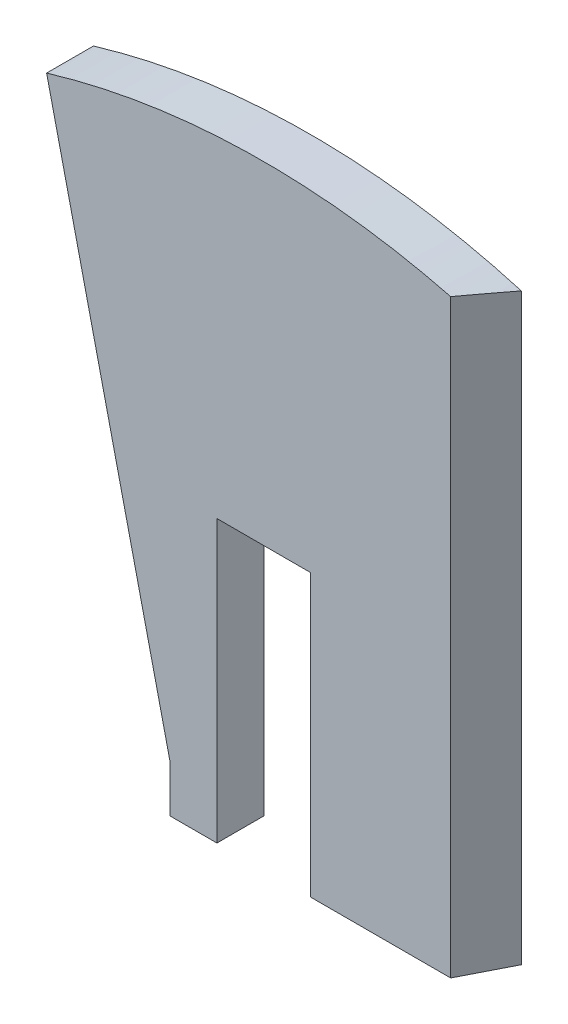
SolidWorks part; units mm, degrees
ref_plane "Front Plane" through (0, 0, 0) normal (0, 0, 1) x (1, 0, 0)
ref_plane "Top Plane" through (0, 0, 0) normal (0, 1, 0) x (1, 0, 0)
ref_plane "Right Plane" through (0, 0, 0) normal (1, 0, 0) x (0, 0, -1)
sketch "Sketch1" plane through (0, 0, 0) normal (0, 0, 1) x (1, 0, 0)
  line L0 (0, 161) -> (0, -161) construction
  line L1 (-46.3607, 154.1807) -> (-20, 40)
  line L2 (-20, 40) -> (-20, 30)
  line L4 (45, 30) -> (45, 40)
  line L5 (45, 40) -> (45, 154.5833)
  line L6 (-20, 30) -> (0, 30)
  line L7 (0, 30) -> (45, 30)
  line L8 (45, 154.5833) -> (0, 30) construction
  arc A0 (45, 154.5833) -> (-46.3607, 154.1807) centre (0, 0) ccw
  dimension "D3" = 322
  dimension "D1" = 30
  dimension "D2" = 20
  dimension "D4" = 10
  dimension "D5" = 45
  dimension "D6" = 13
extrude "Boss-Extrude1" add sketch "Sketch1" along normal mid plane 10
sketch "Sketch2" plane through (0, 0, 5) normal (0, 0, 1) x (1, 0, 0)
  line L0 (-20, 30) -> (45, 30) construction
  line L1 (10, -30) -> (-10, -30)
  line L2 (10, -30) -> (10, 90)
  line L3 (10, 90) -> (-10, 90)
  line L4 (-10, -30) -> (-10, 90)
  line L5 (10, -30) -> (-10, 90) construction
  line L6 (10, 90) -> (-10, -30) construction
  line L7 (-20, 40) -> (-20, 30) construction
  point P0 (0, 30)
  dimension "D1" = 10
  dimension "D2" = 20
  dimension "D3" = 60
extrude "Cut-Extrude1" cut sketch "Sketch2" against normal blind 10
sketch "Sketch3" plane through (0, 30, 0) normal (0, -1, 0) x (1, 0, 0)
  line L4 (45, -5) -> (39.9047, 5)
  line L5 (10, 5) -> (45, 5) construction
  line L6 (39.9047, 5) -> (45, 5)
  line L7 (45, 5) -> (45, -5)
  dimension "D1" = 27
extrude "Cut-Extrude2" cut sketch "Sketch3" against normal through all
